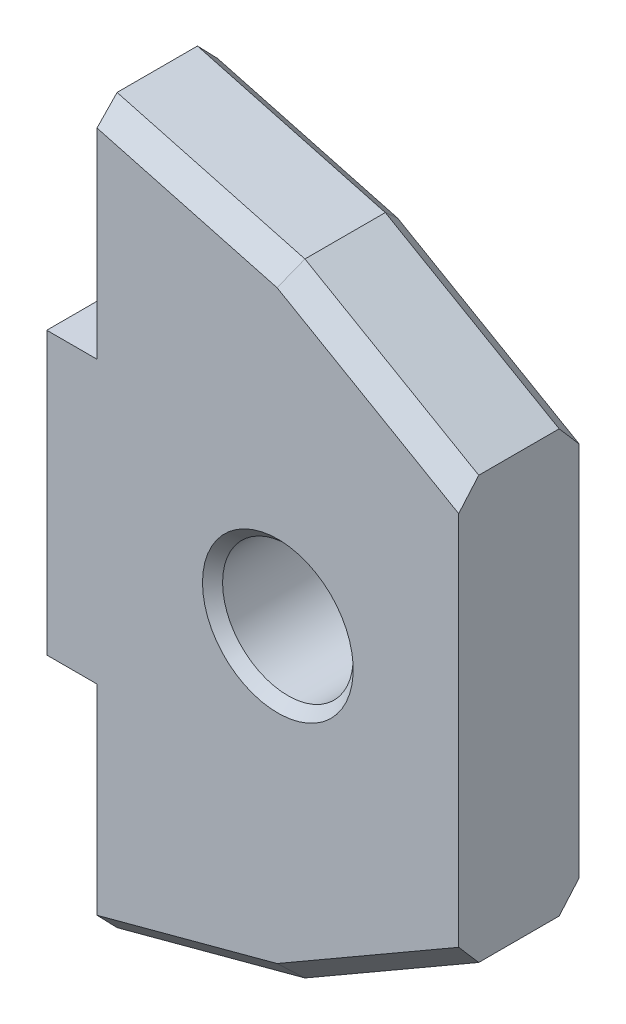
SolidWorks part; units mm, degrees
ref_plane "Front Plane" through (0, 0, 0) normal (0, 0, 1) x (1, 0, 0)
ref_plane "Top Plane" through (0, 0, 0) normal (0, 1, 0) x (1, 0, 0)
ref_plane "Right Plane" through (0, 0, 0) normal (1, 0, 0) x (0, 0, -1)
other "Configuration Table"
sketch "Sketch1" plane through (0, 0, 0) normal (0, 0, 1) x (1, 0, 0)
  line L0 (0, 0) -> (-15.5566, 0) construction
  line L1 (-23, -14) -> (-23, 14)
  line L2 (-23, 14) -> (-18, 14)
  line L3 (-18, 14) -> (-18, 36)
  line L4 (-18, 36) -> (0.6962, 30.9904)
  line L5 (0.6962, 30.9904) -> (18, 21)
  line L6 (18, 21) -> (18, -21)
  line L7 (0.6962, -30.9904) -> (18, -21)
  line L8 (-18, -36) -> (0.6962, -30.9904)
  line L9 (-18, -14) -> (-18, -36)
  line L10 (-23, -14) -> (-18, -14)
  circle A0 centre (0, 0) radius 6.5
  point P13 (18, 0)
  point P18 (-23, 0)
  dimension "D9" = 6.5
  dimension "D1" = 18
  dimension "D2" = 28
  dimension "D3" = 15
  dimension "D4" = 30
  dimension "D5" = 42
  dimension "D6" = 41
  dimension "D7" = 5
  dimension "D8" = 72
extrude "Boss-Extrude1" add sketch "Sketch1" along normal mid plane 12 contours L4 L5 L6 L7 L8 L9 L10 L1 L2 L3 | A0
chamfer "Chamfer1" distance 2 angle 45 8 edges at (9.3481, -25.9952, -6) (-8.6519, -33.4952, -6) (9.3481, -25.9952, 6) (-8.6519, -33.4952, 6) (-8.6519, 33.4952, -6) (9.3481, 25.9952, -6) (9.3481, 25.9952, 6) (-8.6519, 33.4952, 6)
chamfer "Chamfer2" distance 1 angle 45 2 edges at (-6.5, 0, -6) (-6.5, 0, 6)
